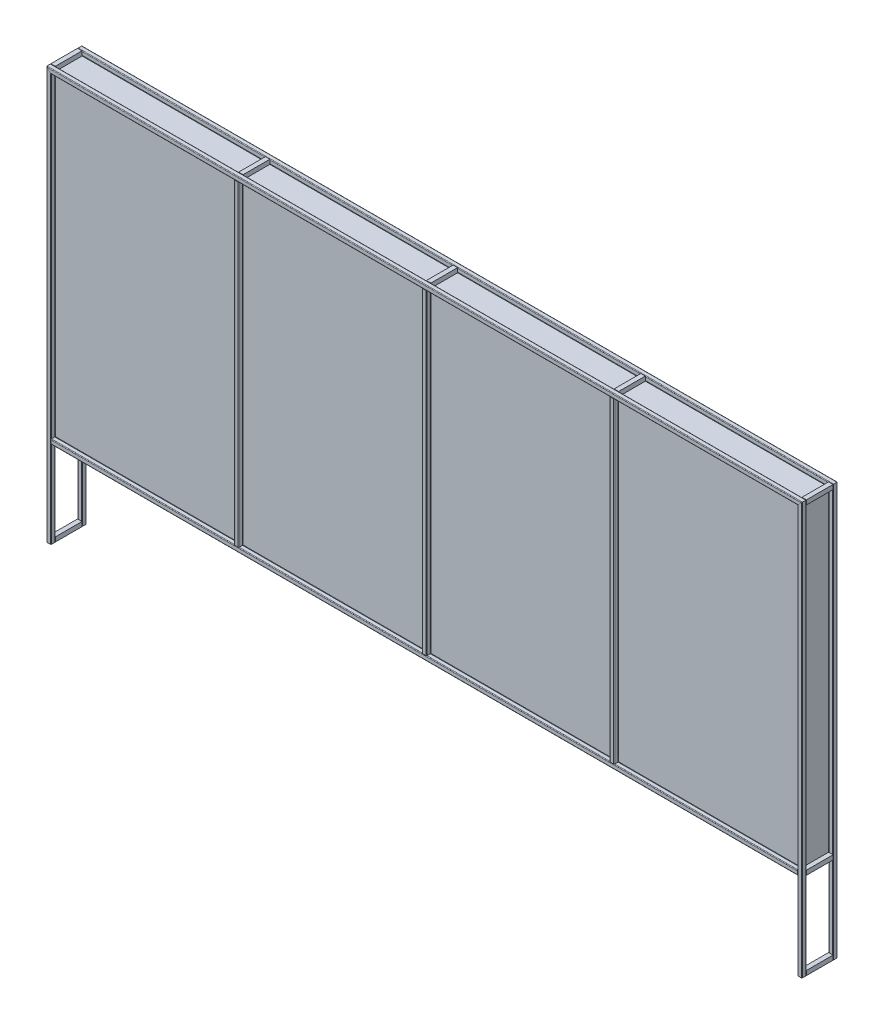
SolidWorks part; units mm, degrees
ref_plane "前视基准面" through (0, 0, 0) normal (0, 0, 1) x (1, 0, 0)
ref_plane "上视基准面" through (0, 0, 0) normal (0, 1, 0) x (1, 0, 0)
ref_plane "右视基准面" through (0, 0, 0) normal (1, 0, 0) x (0, 0, -1)
sketch "草图1" plane through (0, 0, 0) normal (0, 0, 1) x (1, 0, 0)
  line L0 (0, 0) -> (0, 2300) construction
  line L1 (-2107.5, 2300) -> (2107.5, 2300)
  line L2 (-2107.5, 2300) -> (-2107.5, 0)
  line L3 (2107.5, 2300) -> (2107.5, 0)
  line L4 (-2107.5, 500) -> (2107.5, 500)
  line L5 (-1053.75, 2300) -> (-1053.75, 500)
  line L6 (1053.75, 2300) -> (1053.75, 500)
  line L7 (0, 500) -> (0, 2300)
  point P6 (0, 2300)
  dimension "D1" = 4215
  dimension "D2" = 2300
  dimension "D3" = 1800
  dimension "D4" = 1053.75
other "Gb／6728-1986方形空心型钢 025 X 25 X 1.75(1)"
ref_plane "基准面1" through (-2107.5, 2300, 0) normal (0, -1, 0) x (1, 0, 0)
sketch "Sketch1" plane through (-2107.5, 2300, 0) normal (0, -1, 0) x (1, 0, 0)
  line L0 (-9, -10.75) -> (9, -10.75)
  line L1 (-10.75, -9) -> (-10.75, 9)
  line L2 (9, 10.75) -> (-9, 10.75)
  line L3 (10.75, 9) -> (10.75, -9)
  line L4 (-9, -12.5) -> (9, -12.5)
  line L5 (-12.5, -9) -> (-12.5, 9)
  line L6 (9, 12.5) -> (-9, 12.5)
  line L7 (12.5, 9) -> (12.5, -9)
  arc A0 (12.5, 9) -> (9, 12.5) centre (9, 9) ccw
  arc A1 (9, -12.5) -> (12.5, -9) centre (9, -9) ccw
  arc A2 (-12.5, -9) -> (-9, -12.5) centre (-9, -9) ccw
  arc A3 (-9, 12.5) -> (-12.5, 9) centre (-9, 9) ccw
  arc A4 (-9, 10.75) -> (-10.75, 9) centre (-9, 9) ccw
  arc A5 (10.75, 9) -> (9, 10.75) centre (9, 9) ccw
  arc A6 (9, -10.75) -> (10.75, -9) centre (9, -9) ccw
  arc A7 (-10.75, -9) -> (-9, -10.75) centre (-9, -9) ccw
  point P0 (-12.5, 0)
  point P1 (12.5, 0)
  point P2 (0, 12.5)
  point P3 (0, -12.5)
  point P4 (0, 0)
  point P5 (-12.5, -12.5)
  point P6 (12.5, -12.5)
  point P7 (12.5, 12.5)
  point P8 (-12.5, 12.5)
  point P33 (0, 0)
  dimension "D1" = 3.5
  dimension "Thickness" = 1.75
  dimension "V_leg" = 25
pattern_linear "阵列(线性)1" count 2 spacing 175 along (0, 0, -1) of bodies 120 123 121 106 109 108 107
sketch "草图2" plane through (0, 0, -162.5) normal (0, 0, 1) x (1, 0, 0)
  line L0 (-2095, 0) -> (-2095, 2287.5) construction
  line L1 (-2120, 2312.5) -> (-2095, 2312.5)
  line L2 (-2120, 2312.5) -> (-2120, 2287.5)
  line L3 (-2120, 2287.5) -> (-2095, 2287.5)
  line L4 (-2095, 2312.5) -> (-2095, 2287.5)
  line L5 (-2095, 487.5) -> (-2120, 487.5)
  line L6 (-2095, 487.5) -> (-2095, 512.5)
  line L7 (-2095, 512.5) -> (-2120, 512.5)
  line L8 (-2120, 487.5) -> (-2120, 512.5)
  line L9 (2095, 487.5) -> (-2095, 487.5) construction
  line L10 (2095, 512.5) -> (-2095, 512.5) construction
  line L11 (0, 0) -> (0, 1181.8138) construction
  line L12 (-2120, 0) -> (-2095, 0)
  line L13 (-2120, 0) -> (-2120, 25)
  line L14 (-2120, 25) -> (-2095, 25)
  line L15 (-2095, 0) -> (-2095, 25)
  line L16 (2095, 0) -> (2095, 25)
  line L17 (2120, 25) -> (2095, 25)
  line L18 (2120, 0) -> (2120, 25)
  line L19 (2120, 0) -> (2095, 0)
  line L20 (2120, 487.5) -> (2120, 512.5)
  line L21 (2095, 512.5) -> (2120, 512.5)
  line L22 (2095, 487.5) -> (2095, 512.5)
  line L23 (2095, 487.5) -> (2120, 487.5)
  line L24 (2095, 2312.5) -> (2095, 2287.5)
  line L25 (2120, 2287.5) -> (2095, 2287.5)
  line L26 (2120, 2312.5) -> (2120, 2287.5)
  line L27 (2120, 2312.5) -> (2095, 2312.5)
  line L28 (-2120, 2312.5) -> (2120, 2312.5) construction
  line L29 (-1066.25, 2287.5) -> (-1041.25, 2287.5)
  line L30 (-1066.25, 2287.5) -> (-1066.25, 2312.5)
  line L31 (-1066.25, 2312.5) -> (-1041.25, 2312.5)
  line L32 (-1041.25, 2287.5) -> (-1041.25, 2312.5)
  line L33 (-2095, 2287.5) -> (2095, 2287.5) construction
  line L34 (-1041.25, 2287.5) -> (-1044.75, 2287.5) construction
  line L35 (-1041.25, 512.5) -> (-1041.25, 2287.5) construction
  line L36 (-1066.25, 512.5) -> (-1041.25, 512.5)
  line L37 (-1066.25, 512.5) -> (-1066.25, 487.5)
  line L38 (-1066.25, 487.5) -> (-1041.25, 487.5)
  line L39 (-1041.25, 512.5) -> (-1041.25, 487.5)
  line L40 (-1066.25, 512.5) -> (-1066.25, 2287.5) construction
  line L41 (1041.25, 512.5) -> (1041.25, 487.5)
  line L42 (1066.25, 487.5) -> (1041.25, 487.5)
  line L43 (1066.25, 512.5) -> (1066.25, 487.5)
  line L44 (1066.25, 512.5) -> (1041.25, 512.5)
  line L45 (1041.25, 2287.5) -> (1041.25, 2312.5)
  line L46 (1066.25, 2312.5) -> (1041.25, 2312.5)
  line L47 (1066.25, 2287.5) -> (1066.25, 2312.5)
  line L48 (1066.25, 2287.5) -> (1041.25, 2287.5)
  line L49 (12.5, 512.5) -> (12.5, 2287.5) construction
  line L50 (-12.5, 512.5) -> (12.5, 512.5)
  line L51 (-12.5, 512.5) -> (-12.5, 487.5)
  line L52 (-12.5, 487.5) -> (12.5, 487.5)
  line L53 (12.5, 512.5) -> (12.5, 487.5)
  line L55 (-12.5, 2287.5) -> (12.5, 2287.5)
  line L56 (-12.5, 2287.5) -> (-12.5, 2312.5)
  line L57 (-12.5, 2312.5) -> (12.5, 2312.5)
  line L58 (12.5, 2287.5) -> (12.5, 2312.5)
extrude "凸台-拉伸1" add sketch "草图2" along normal up to surface (150 mm away) separate body up to face at (0, 2300, -12.5)
sketch "草图3" plane through (0, 0, -12.5) normal (0, 0, -1) x (-1, 0, 0)
  line L1 (-2095, 2287.5) -> (-1066.25, 2287.5)
  line L2 (-2095, 2287.5) -> (-2095, 512.5)
  line L3 (-2095, 512.5) -> (-1066.25, 512.5)
  line L4 (-1066.25, 2287.5) -> (-1066.25, 512.5)
extrude "凸台-拉伸2" add sketch "草图3" along normal up to surface (150 mm away) up to face at (2107.5, 1150, -162.5)
pattern_linear "阵列(线性)3" count 4 spacing 1053.75 along (-1, 0, 0) of bodies 133
